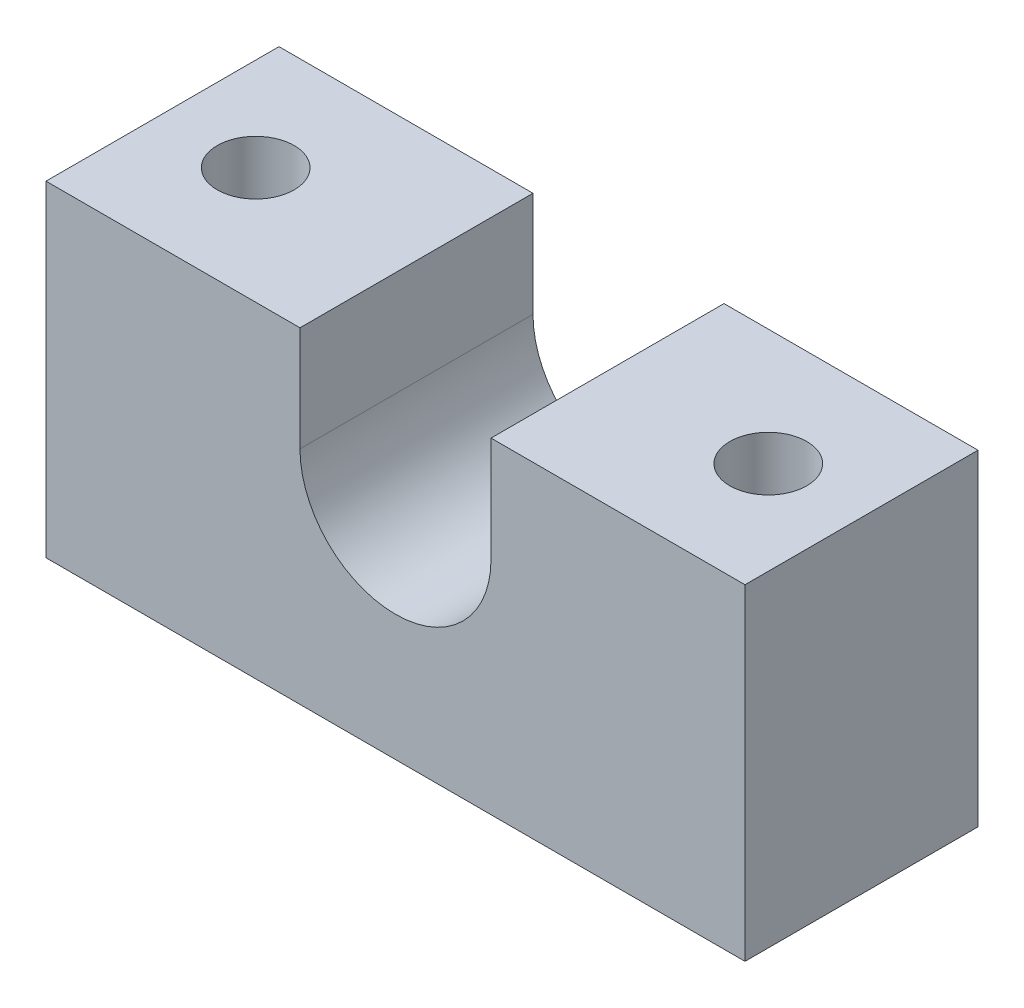
from build123d import *

# Parameters (mm, degrees)
SKETCH1_W           = 30
SKETCH1_H           = 14
BOSS_EXTRUDE1_DEPTH = 5
CUT_EXTRUDE1_DEPTH  = 20.339079606
M4_TAPPED_HOLE1_D   = 3.3


with BuildPart() as part:
    # Sketch1 → Boss-Extrude1 (new, symmetric)
    with BuildSketch(Plane.XY):
        Rectangle(SKETCH1_W, SKETCH1_H)
    extrude(amount=BOSS_EXTRUDE1_DEPTH, both=True)

    # Sketch2 → Cut-Extrude1 (cut, through all)
    with BuildSketch(Plane.XY.offset(5)):
        with BuildLine():
            Line((4.1, 7), (4.1, 2.5))
            ThreePointArc((4.1, 2.5), (0, -1.6), (-4.1, 2.5))
            Line((-4.1, 2.5), (-4.1, 7))
            ThreePointArc((-4.1, 7), (0, 11.1), (4.1, 7))
        make_face()
    extrude(amount=-CUT_EXTRUDE1_DEPTH, mode=Mode.SUBTRACT)

    # M4 Tapped Hole1 (through all)
    with Locations(Plane(origin=(0, 7, 0), x_dir=(1, 0, 0), z_dir=(0, 1, 0))):
        with Locations((-11, 0), (11, 0)):
            Hole(M4_TAPPED_HOLE1_D / 2)


solid = part.part
